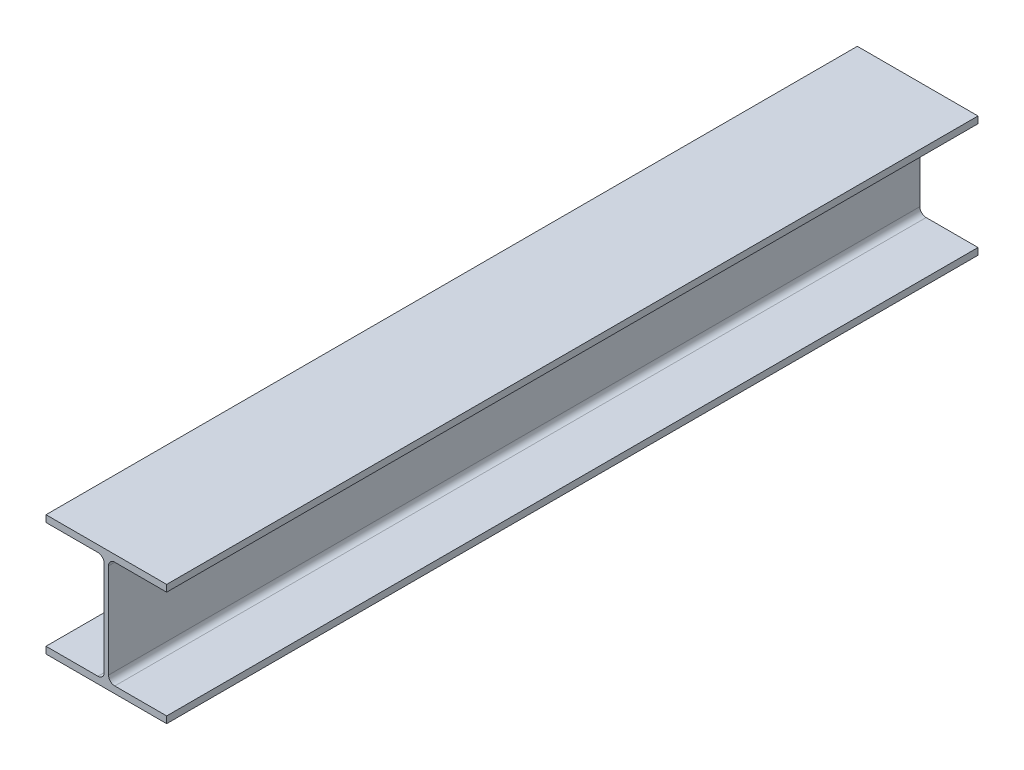
from build123d import *

# Parameters (mm, degrees)
BOSS_EXTRUDE1_DEPTH = 1681


with BuildPart() as part:
    # Sketch1 → Boss-Extrude1 (new body)
    with BuildSketch(Plane.XY):
        with BuildLine():
            Line((0, 0), (250, 0))
            Line((250, 0), (250, 14))
            Line((250, 14), (142.5, 14))
            ThreePointArc((142.5, 14), (133.307611845, 17.807611845), (129.5, 27))
            Line((129.5, 27), (129.5, 223))
            ThreePointArc((129.5, 223), (133.307611845, 232.192388155), (142.5, 236))
            Line((142.5, 236), (250, 236))
            Line((250, 236), (250, 250))
            Line((250, 250), (0, 250))
            Line((0, 250), (0, 236))
            Line((0, 236), (107.5, 236))
            ThreePointArc((107.5, 236), (116.692388155, 232.192388155), (120.5, 223))
            Line((120.5, 223), (120.5, 27))
            ThreePointArc((120.5, 27), (116.692388155, 17.807611845), (107.5, 14))
            Line((107.5, 14), (0, 14))
            Line((0, 14), (0, 0))
        make_face()
    extrude(amount=BOSS_EXTRUDE1_DEPTH)


solid = part.part
